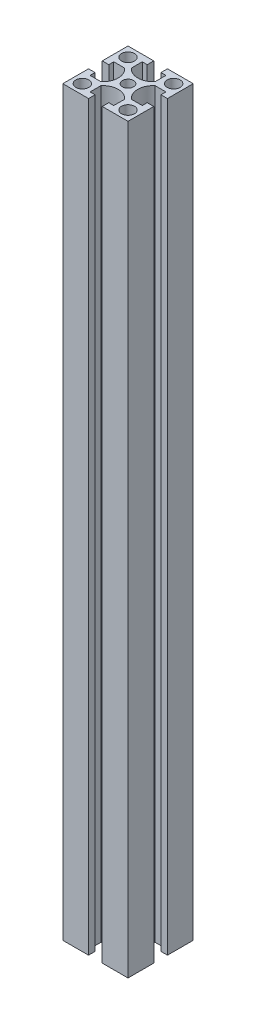
from build123d import *

# Parameters (mm, degrees)
SKETCH_3_R     = 4
SKETCH_3_R_2   = 3.4
EF4040_1_DEPTH = 455


with BuildPart() as part:
    # 草圖3 → 東野鋁型材 EF4040(1) (new body)
    with BuildSketch(Plane(origin=(0, 0, 0), x_dir=(-1, 0, 0), z_dir=(0, 1, 0))):
        with BuildLine():
            Line((-20, -20), (-4.2, -20))
            Line((-4.2, -20), (-4.2, -16))
            Line((-4.2, -16), (-7.25, -16))
            Line((-7.25, -16), (-7.25, -9.360985421))
            ThreePointArc((-7.25, -9.360985421), (0, -6), (7.25, -9.360985421))
            Line((7.25, -9.360985421), (7.25, -16))
            Line((7.25, -16), (4.2, -16))
            Line((4.2, -16), (4.2, -20))
            Line((4.2, -20), (20, -20))
            Line((20, -20), (20, -4.2))
            Line((20, -4.2), (16, -4.2))
            Line((16, -4.2), (16, -7.25))
            Line((16, -7.25), (9.360985421, -7.25))
            ThreePointArc((9.360985421, -7.25), (6, 0), (9.360985421, 7.25))
            Line((9.360985421, 7.25), (16, 7.25))
            Line((16, 7.25), (16, 4.2))
            Line((16, 4.2), (20, 4.2))
            Line((20, 4.2), (20, 20))
            Line((20, 20), (4.2, 20))
            Line((4.2, 20), (4.2, 16))
            Line((4.2, 16), (7.25, 16))
            Line((7.25, 16), (7.25, 9.360985421))
            ThreePointArc((7.25, 9.360985421), (0, 6), (-7.25, 9.360985421))
            Line((-7.25, 9.360985421), (-7.25, 16))
            Line((-7.25, 16), (-4.2, 16))
            Line((-4.2, 16), (-4.2, 20))
            Line((-4.2, 20), (-20, 20))
            Line((-20, 20), (-20, 4.2))
            Line((-20, 4.2), (-16, 4.2))
            Line((-16, 4.2), (-16, 7.25))
            Line((-16, 7.25), (-9.360985421, 7.25))
            ThreePointArc((-9.360985421, 7.25), (-6, 0), (-9.360985421, -7.25))
            Line((-9.360985421, -7.25), (-16, -7.25))
            Line((-16, -7.25), (-16, -4.2))
            Line((-16, -4.2), (-20, -4.2))
            Line((-20, -4.2), (-20, -20))
        make_face()
        with Locations((-13.999999649, -13.999999649)):
            Circle(SKETCH_3_R, mode=Mode.SUBTRACT)
        Circle(SKETCH_3_R_2, mode=Mode.SUBTRACT)
        with Locations((14.00000014, -13.999999158)):
            Circle(SKETCH_3_R, mode=Mode.SUBTRACT)
        with Locations((-13.999999649, 14.000000351)):
            Circle(SKETCH_3_R, mode=Mode.SUBTRACT)
        with Locations((13.999999158, 14.000000842)):
            Circle(SKETCH_3_R, mode=Mode.SUBTRACT)
    extrude(amount=EF4040_1_DEPTH)


solid = part.part
